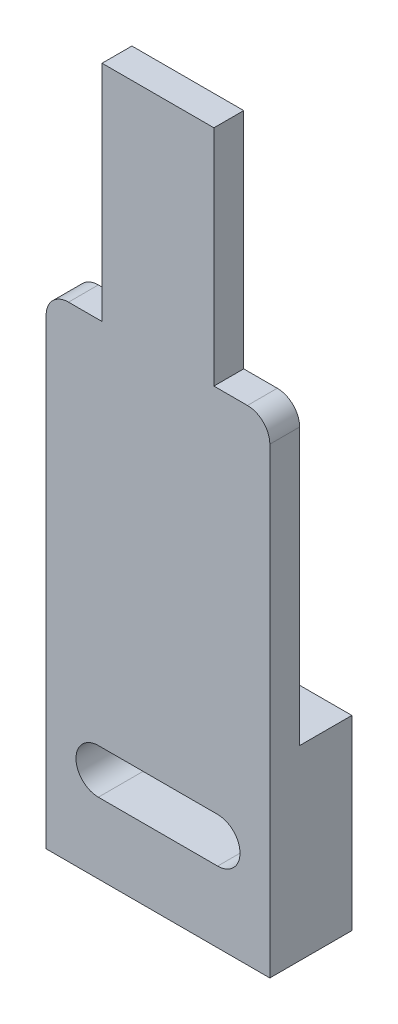
from build123d import *

# Parameters (mm, degrees)
EXTRUDE_1_DEPTH = 7
SKETCH_2_W      = 30
SKETCH_2_H      = 65
EXTRUDE_2_DEPTH = 4
FILLET_1_R      = 3
SKETCH_3_W      = 15
SKETCH_3_H      = 30
EXTRUDE_3_DEPTH = 4


with BuildPart() as part:
    # 草图1 → 凸台-拉伸1 (new body)
    with BuildSketch(Plane.XY):
        Polygon((0, 0), (-15, 0), (-15, 25), (15, 25), (15, 0), align=None)
        with BuildLine():
            Line((-8, 15.5), (8, 15.5))
            ThreePointArc((8, 15.5), (11, 12.5), (8, 9.5))
            Line((8, 9.5), (-8, 9.5))
            ThreePointArc((-8, 9.5), (-11, 12.5), (-8, 15.5))
        make_face(mode=Mode.SUBTRACT)
    extrude(amount=EXTRUDE_1_DEPTH)

    # 草图2 → 凸台-拉伸2 (add)
    with BuildSketch(Plane.XY.offset(7)):
        with Locations((0, 32.5)):
            Rectangle(SKETCH_2_W, SKETCH_2_H)
        with BuildLine():
            Line((-8, 9.5), (8, 9.5))
            ThreePointArc((8, 9.5), (11, 12.5), (8, 15.5))
            Line((8, 15.5), (-8, 15.5))
            ThreePointArc((-8, 15.5), (-11, 12.5), (-8, 9.5))
        make_face(mode=Mode.SUBTRACT)
    extrude(amount=EXTRUDE_2_DEPTH)

    # 圆角1
    fillet_1_edges = [part.edges().sort_by_distance(p)[0] for p in [
        (-15, 65, 9),
        (15, 65, 9),
    ]]
    fillet(fillet_1_edges, radius=FILLET_1_R)

    # 草图3 → 凸台-拉伸3 (add)
    with BuildSketch(Plane.XY.offset(11)):
        with Locations((0, 80)):
            Rectangle(SKETCH_3_W, SKETCH_3_H)
    extrude(amount=-EXTRUDE_3_DEPTH)


solid = part.part
